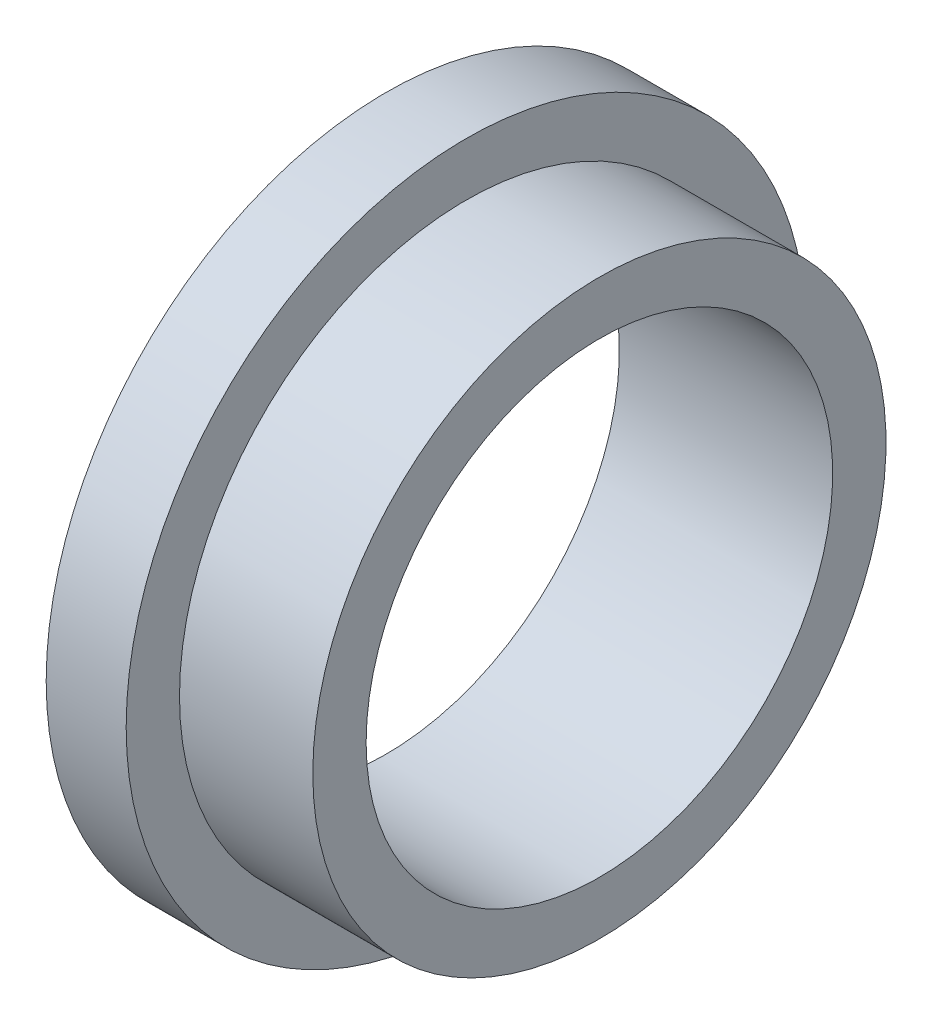
SolidWorks part; units mm, degrees
ref_plane "Front" through (0, 0, 0) normal (0, 0, 1) x (1, 0, 0)
ref_plane "Top" through (0, 0, 0) normal (0, 1, 0) x (1, 0, 0)
ref_plane "Right" through (0, 0, 0) normal (1, 0, 0) x (0, 0, -1)
sketch "Sketch1" plane through (0, 0, 0) normal (0, 0, 1) x (1, 0, 0)
  line L0 (-17.2118, 17.5) -> (-5.3427, 17.5)
  line L1 (-5.3427, 17.5) -> (-5.3427, 21.5)
  line L2 (-5.3427, 21.5) -> (-15.3427, 21.5)
  line L3 (-15.3427, 21.5) -> (-15.3427, 25.5)
  line L4 (-15.3427, 25.5) -> (-21.3427, 25.5)
  line L5 (-21.3427, 25.5) -> (-21.3427, 17.5)
  line L6 (-21.3427, 17.5) -> (-17.2118, 17.5)
  line L7 (-21.3427, 0) -> (0, 0) construction
  line L8 (0, 0) -> (40.2602, 0) construction
  dimension "D1" = 17.5
  dimension "D2" = 4
  dimension "D3" = 8
  dimension "D4" = 6
  dimension "D5" = 16
revolve "Revolve1" add sketch "Sketch1" angle 360 about L8
